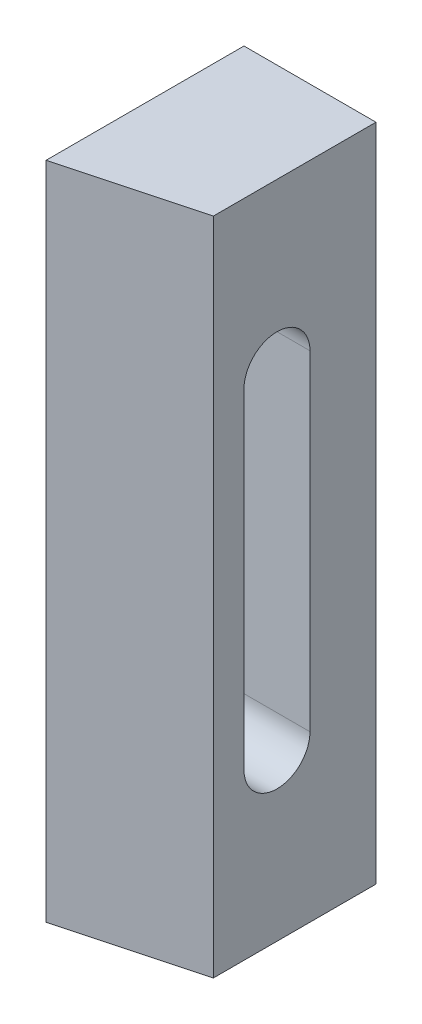
from build123d import *

# Parameters (mm, degrees)
SKETCH1_W           = 60
SKETCH1_H           = 200
BOSS_EXTRUDE1_DEPTH = 20
CUT_EXTRUDE1_DEPTH  = 210.761769634


with BuildPart() as part:
    # Sketch1 → Boss-Extrude1 (new, symmetric)
    with BuildSketch(Plane(origin=(0, 0, 0), x_dir=(0, 0, -1), z_dir=(1, 0, 0))):
        with Locations((30, 100)):
            Rectangle(SKETCH1_W, SKETCH1_H)
        with BuildLine():
            Line((20, 50), (20, 150))
            ThreePointArc((20, 150), (30, 160), (40, 150))
            Line((40, 150), (40, 50))
            ThreePointArc((40, 50), (30, 40), (20, 50))
        make_face(mode=Mode.SUBTRACT)
    extrude(amount=BOSS_EXTRUDE1_DEPTH, both=True)

    # Sketch3 → Cut-Extrude1 (cut, through all)
    with BuildSketch(Plane.XZ):
        Polygon((-20, 0), (20, -10.717967697), (20, 0), align=None)
    extrude(amount=-CUT_EXTRUDE1_DEPTH, mode=Mode.SUBTRACT)


solid = part.part
